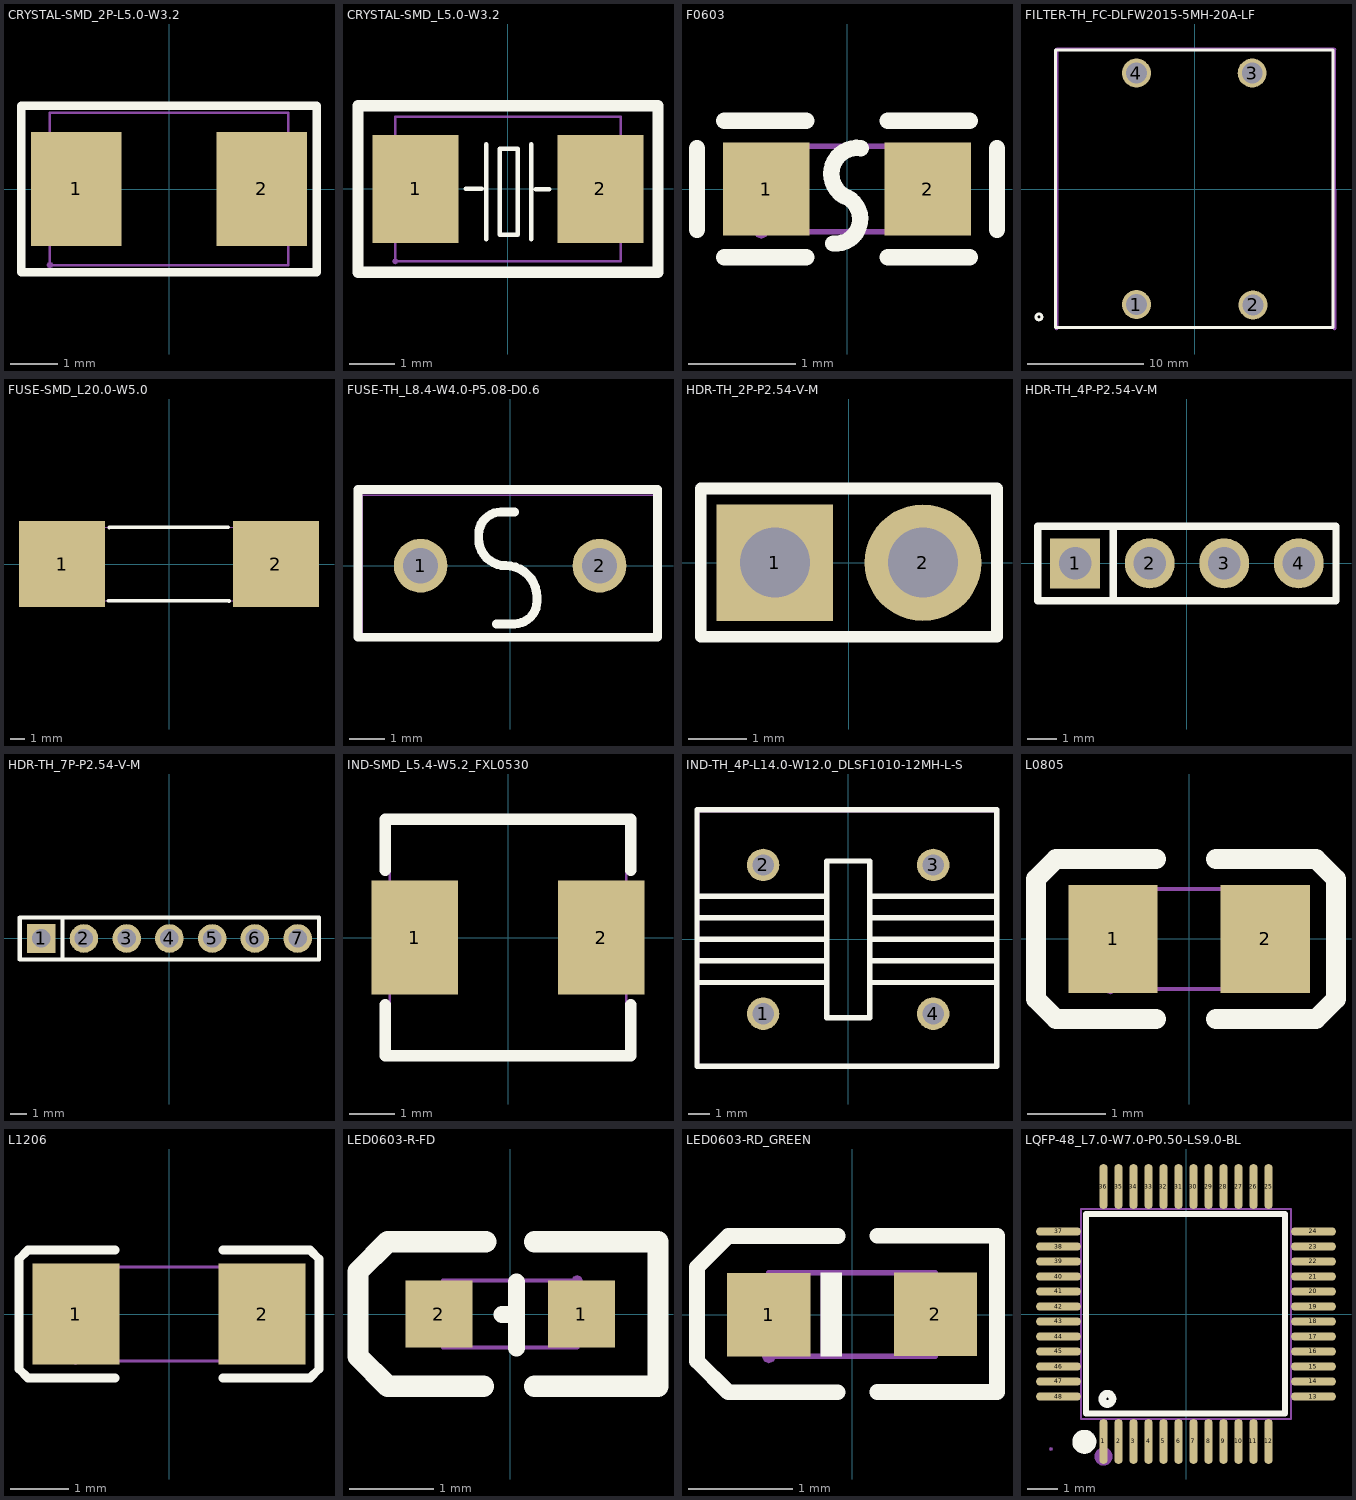
[diagram p0: the footprints below, top view; thin cyan lines are the x and y axes]
# Altium footprint library MISC84429-11.PcbLib: 64 footprints (part 2 of 4)
Each footprint in its own frame and in the unit in brackets; x right, y up, seen from the top. Pads: shape width x height; smd on the part's side, far side on the other; paste and mask are expansions set on the pad; w line width, h text height; cw(c..) or ccw(c..) is an arc to the next point about the centre after c.

## CRYSTAL-SMD_2P-L5.0-W3.2 [mm]
pads (2):
  rect 1.9x2.4 smd: 1(-1.95,0) 2(1.95,0)
Top Overlay:
  lines w0.18: -3.099,-1.75 3.099,-1.75 3.099,1.75 -3.099,1.75 -3.099,1.4 -3.099,-1.75
Mechanical 2:
  region: -2.435,-1.6 -2.454,-1.646 -2.5,-1.665 -2.546,-1.646 -2.565,-1.6 -2.546,-1.554 -2.5,-1.535 -2.454,-1.554
  region: 1.2,-1 1.2,1 2.5,1 2.5,-1
  region: -1.2,-1 -1.2,1 -2.5,1 -2.5,-1
  lines w0.051: -2.5,-1.6 -2.5,1.6 2.5,1.6 2.5,-1.6 -2.5,-1.6

## CRYSTAL-SMD_L5.0-W3.2 [mm]
pads (2):
  rect 1.9x2.4 smd: 1(-2.05,0) 2(2.05,0)
Top Overlay:
  lines w0.1: -0.94,0 -0.584,0 ; -0.483,-1.109 -0.483,0.991 ; 0.517,-1.109 0.517,0.991 ; 0.617,-0.009 0.917,-0.009 ; -0.183,-1.009 -0.183,0.89 0.217,0.89 0.217,-1.009 -0.183,-1.009
  lines w0.254: -3.325,-1.85 3.325,-1.85 3.325,-0.7 3.325,0.7 3.325,1.85 -3.325,1.85 -3.325,0.7 -3.325,-0.7 -3.325,-1.85
Mechanical 2:
  region: -2.435,-1.6 -2.454,-1.646 -2.5,-1.665 -2.546,-1.646 -2.565,-1.6 -2.546,-1.554 -2.5,-1.535 -2.454,-1.554
  region: -2.4,1 -1.3,1 -1.3,-1 -2.4,-1
  region: 1.3,1 2.4,1 2.4,-1 1.3,-1
  lines w0.051: -2.5,-1.6 -2.5,1.6 2.5,1.6 2.5,-1.6 -2.5,-1.6

## F0603 [mm]
pads (2):
  rect 0.806x0.864 smd paste-100 mask+0.051: 1(-0.753,0) 2(0.753,0)
Top Overlay:
  lines w0.152: -1.397,-0.381 -1.397,0.381 ; -1.143,-0.635 -0.381,-0.635 ; -1.143,0.635 -0.381,0.635 ; -0.127,-0.508 ccw(c-0.107,-0.28) -0.031,-0.063 ; -0.032,-0.064 cw(c0.096,0.142) 0.127,0.381 ; 0.381,-0.635 1.143,-0.635 ; 0.381,0.635 1.143,0.635 ; 1.397,-0.381 1.397,0.381
Top Paste:
  region: 0.315,-0.138 0.315,0.138 0.589,0.432 1.092,0.432 1.156,0.368 1.156,-0.368 1.092,-0.432 0.589,-0.432
  region: -0.315,-0.138 -0.315,0.138 -0.589,0.432 -1.092,0.432 -1.156,0.368 -1.156,-0.368 -1.092,-0.432 -0.589,-0.432
Mechanical 2:
  region: -0.735,-0.4 -0.754,-0.446 -0.8,-0.465 -0.846,-0.446 -0.865,-0.4 -0.846,-0.354 -0.8,-0.335 -0.754,-0.354
  region: -0.8,-0.4 -0.8,0.4 -0.5,0.4 -0.5,-0.4
  region: 0.8,-0.4 0.8,0.4 0.5,0.4 0.5,-0.4
  lines w0.051: -0.8,-0.4 -0.8,0.4 0.8,0.4 0.8,-0.4 -0.8,-0.4

## FILTER-TH_FC-DLFW2015-5MH-20A-LF [mm]
pads (4):
  round 2.5 hole 1.8 paste+0 mask-0.3: 1(-5.04,-9.983) 2(5.04,-10.016) 3(4.96,10.016) 4(-5.04,10.016)
Top Overlay:
  circle w0.254: c-13.462,-11.049 r0.254
  lines w0.254: -12.04,-11.983 11.96,-11.983 11.96,12.016 -12.04,12.016 -12.04,-11.983
Mechanical 1:
  region: -12.065,-12.065 -12.075,12.065 -12.035,12.162 -11.938,12.202 -11.938,12.192 12.065,12.202 12.162,12.162 12.202,12.065 12.192,12.065 12.202,-12.065 12.162,-12.162 12.065,-12.202 11.968,-12.162 11.928,-12.065 11.938,-12.065 11.938,11.938 -11.811,11.938 -11.801,-12.065 -11.841,-12.162 -11.938,-12.202 -12.035,-12.162 -12.075,-12.065
Mechanical 2:
  region: -4.284,-9.983 -4.309,-10.179 -4.385,-10.362 -4.505,-10.518 -4.662,-10.639 -4.844,-10.714 -5.04,-10.74 -5.236,-10.714 -5.418,-10.639 -5.575,-10.518 -5.695,-10.362 -5.771,-10.179 -5.796,-9.983 -5.771,-9.788 -5.695,-9.605 -5.575,-9.449 -5.418,-9.328 -5.236,-9.253 -5.04,-9.227 -4.844,-9.253 -4.662,-9.328 -4.505,-9.449 -4.385,-9.605 -4.309,-9.788
  region: 5.796,-10.016 5.771,-10.212 5.695,-10.395 5.575,-10.551 5.418,-10.672 5.236,-10.747 5.04,-10.773 4.844,-10.747 4.662,-10.672 4.505,-10.551 4.385,-10.395 4.309,-10.212 4.284,-10.016 4.309,-9.821 4.385,-9.638 4.505,-9.482 4.662,-9.361 4.844,-9.286 5.04,-9.26 5.236,-9.286 5.418,-9.361 5.575,-9.482 5.695,-9.638 5.771,-9.821
  region: 5.716,10.016 5.691,9.821 5.615,9.638 5.495,9.482 5.338,9.361 5.156,9.286 4.96,9.26 4.764,9.286 4.582,9.361 4.425,9.482 4.305,9.638 4.229,9.821 4.204,10.016 4.229,10.212 4.305,10.395 4.425,10.551 4.582,10.672 4.764,10.747 4.96,10.773 5.156,10.747 5.338,10.672 5.495,10.551 5.615,10.395 5.691,10.212
  region: -4.284,10.016 -4.309,9.821 -4.385,9.638 -4.505,9.482 -4.662,9.361 -4.844,9.286 -5.04,9.26 -5.236,9.286 -5.418,9.361 -5.575,9.482 -5.695,9.638 -5.771,9.821 -5.796,10.016 -5.771,10.212 -5.695,10.395 -5.575,10.551 -5.418,10.672 -5.236,10.747 -5.04,10.773 -4.844,10.747 -4.662,10.672 -4.505,10.551 -4.385,10.395 -4.309,10.212
  region: -11.935,-12 -11.954,-12.046 -12,-12.065 -12.046,-12.046 -12.065,-12 -12.046,-11.954 -12,-11.935 -11.954,-11.954
  lines w0.051: -12,-12 -12,12 12,12 12,-12 -12,-12

## FUSE-SMD_L20.0-W5.0 [mm]
pads (2):
  rect 6x6 smd: 1(-7.45,0) 2(7.45,0)
Top Overlay:
  lines w0.254: -4.219,-2.561 4.175,-2.58 ; -4.167,2.54 4.139,2.549
Mechanical 2:
  region: -9.935,-2.6 -9.954,-2.646 -10,-2.665 -10.046,-2.646 -10.065,-2.6 -10.046,-2.554 -10,-2.535 -9.954,-2.554
  region: 4.9,-2.6 4.9,2.6 10,2.6 10,-2.6
  region: -4.9,2.6 -4.9,-2.6 -10,-2.6 -10,2.6
  lines w0.051: -10,-2.56 10,-2.56 10,2.56 -10,2.56 -10,-2.56

## FUSE-TH_L8.4-W4.0-P5.08-D0.6 [mil]
pads (2):
  round 60 hole 39.37 paste+0 mask-8.35: 1(-100,0) 2(100,0)
Top Overlay:
  lines w10: -15,-65 5,-65 ccw(c5,-40) 30,-40 30,-35 ccw(c-5,-35) -5,0 cw(c-5,30) -35,30 -35,35 cw(c-10,35) -10,60 5,60 ; -170,-80 165,-80 165,85 -170,85 -170,-80
Mechanical 2:
  region: -162.79,-78.74 -163.54,-80.55 -165.35,-81.3 -167.16,-80.55 -167.91,-78.74 -167.16,-76.93 -165.35,-76.18 -163.54,-76.93
  region: 112.05,0 111.13,-4.61 108.52,-8.52 104.61,-11.13 100,-12.05 95.39,-11.13 91.48,-8.52 88.87,-4.61 87.95,0 88.87,4.61 91.48,8.52 95.39,11.13 100,12.05 104.61,11.13 108.52,8.52 111.13,4.61
  region: -87.95,0 -88.87,-4.61 -91.48,-8.52 -95.39,-11.13 -100,-12.05 -104.61,-11.13 -108.52,-8.52 -111.13,-4.61 -112.05,0 -111.13,4.61 -108.52,8.52 -104.61,11.13 -100,12.05 -95.39,11.13 -91.48,8.52 -88.87,4.61
  lines w2: -165.35,-78.74 -165.35,78.74 165.35,78.74 165.35,-78.74 -165.35,-78.74

## HDR-TH_2P-P2.54-V-M [mm]
pads (2):
  rect 2x2 hole 1.2: 1(-1.27,0)
  round 2 hole 1.2: 2(1.27,0)
Top Overlay:
  lines w0.203: -2.54,-1.27 2.54,-1.27 2.54,1.27 -0.635,1.27 -2.54,1.27 -2.54,-1.27
Mechanical 2:
  region: -2.475,-1.25 -2.494,-1.296 -2.54,-1.315 -2.586,-1.296 -2.605,-1.25 -2.586,-1.204 -2.54,-1.185 -2.494,-1.204
  region: 0.95,0.32 1.59,0.32 1.59,-0.32 0.95,-0.32
  region: -1.59,0.32 -0.95,0.32 -0.95,-0.32 -1.59,-0.32
  lines w0.051: -2.54,-1.25 -2.54,1.25 2.54,1.25 2.54,-1.25 -2.54,-1.25

## HDR-TH_4P-P2.54-V-M [mm]
pads (4):
  rect 1.7x1.7 hole 1.1: 1(-3.81,0)
  round 1.7 hole 1.1: 2(-1.27,0) 3(1.27,0) 4(3.81,0)
Top Overlay:
  lines w0.254: -2.516,-1.27 -2.516,1.27 ; -2.516,1.27 5.08,1.27 5.08,-1.27 -5.08,-1.27 -5.08,1.27 -2.516,1.27
Mechanical 2:
  region: -5.015,-1.25 -5.034,-1.296 -5.08,-1.315 -5.126,-1.296 -5.145,-1.25 -5.126,-1.204 -5.08,-1.185 -5.034,-1.204
  region: -4.13,0.32 -3.49,0.32 -3.49,-0.32 -4.13,-0.32
  region: -1.59,0.32 -0.95,0.32 -0.95,-0.32 -1.59,-0.32
  region: 0.95,0.32 1.59,0.32 1.59,-0.32 0.95,-0.32
  region: 3.49,0.32 4.13,0.32 4.13,-0.32 3.49,-0.32
  lines w0.051: -5.08,-1.25 -5.08,1.25 5.08,1.25 5.08,-1.25 -5.08,-1.25

## HDR-TH_7P-P2.54-V-M [mm]
pads (7):
  rect 1.7x1.7 hole 1.1: 1(-7.62,0)
  round 1.7 hole 1.1: 2(-5.08,0) 3(-2.54,0) 4(0,0) 5(2.54,0) 6(5.08,0) 7(7.62,0)
Top Overlay:
  lines w0.254: -6.35,-1.25 -6.35,1.25 ; -8.89,-1.25 8.89,-1.25 8.89,1.25 -8.89,1.25 -8.89,-1.25
Mechanical 2:
  region: -8.81,-1.25 -8.829,-1.296 -8.875,-1.315 -8.921,-1.296 -8.94,-1.25 -8.921,-1.204 -8.875,-1.185 -8.829,-1.204
  region: 7.3,0.32 7.94,0.32 7.94,-0.32 7.3,-0.32
  region: 4.76,0.32 5.4,0.32 5.4,-0.32 4.76,-0.32
  region: 2.22,0.32 2.86,0.32 2.86,-0.32 2.22,-0.32
  region: -0.32,0.32 0.32,0.32 0.32,-0.32 -0.32,-0.32
  region: -2.86,0.32 -2.22,0.32 -2.22,-0.32 -2.86,-0.32
  region: -5.4,0.32 -4.76,0.32 -4.76,-0.32 -5.4,-0.32
  region: -7.94,0.32 -7.3,0.32 -7.3,-0.32 -7.94,-0.32
  lines w0.051: -8.89,-1.25 -8.89,1.25 8.89,1.25 8.89,-1.25 -8.89,-1.25

## IND-SMD_L5.4-W5.2_FXL0530 [mm]
pads (2):
  rect 1.9x2.5 smd: 1(-2.05,0) 2(2.05,0)
Top Overlay:
  lines w0.254: -2.7,-1.481 -2.7,-2.6 2.7,-2.6 2.7,-1.481 ; -2.7,1.481 -2.7,2.6 2.7,2.6 2.7,1.481
Mechanical 2:
  region: -2.635,-2.6 -2.654,-2.646 -2.7,-2.665 -2.746,-2.646 -2.765,-2.6 -2.746,-2.554 -2.7,-2.535 -2.654,-2.554
  region: -2.7,1.1 -1.5,1.1 -1.5,-1.1 -2.7,-1.1
  region: 2.7,-1.1 1.5,-1.1 1.5,1.1 2.7,1.1
  lines w0.051: -2.6,-2.6 2.6,-2.6 2.6,2.6 -2.6,2.6 -2.6,-2.6

## IND-TH_4P-L14.0-W12.0_DLSF1010-12MH-L-S [mm]
pads (4):
  round 1.524 hole 1 paste+0 mask-0.212: 1(-4,-3.5) 2(-4,3.5) 3(4,3.5) 4(4,-3.5)
Top Overlay:
  lines w0.254: -7.112,0 -1.016,0 ; -6.985,-2.032 -1.016,-2.032 ; -6.985,-1.016 -1.016,-1.016 ; -6.985,1.016 -1.016,1.016 ; -6.985,2.032 -1.016,2.032 ; 1.016,-2.032 6.985,-2.032 ; 1.016,-1.016 6.985,-1.016 ; 1.016,0 6.731,0 6.985,0 ; 1.016,1.016 6.858,1.016 ; 1.016,2.032 6.985,2.032 ; -7.112,-5.969 6.985,-5.969 6.985,6.096 -7.112,6.096 -7.112,-5.969 ; -1.016,-3.683 1.016,-3.683 1.016,3.683 -1.016,3.683 -1.016,-3.683
Mechanical 2:
  region: -6.935,-6 -6.954,-6.046 -7,-6.065 -7.046,-6.046 -7.065,-6 -7.046,-5.954 -7,-5.935 -6.954,-5.954
  region: 4.306,-3.5 4.283,-3.617 4.216,-3.716 4.117,-3.783 4,-3.806 3.883,-3.783 3.784,-3.716 3.717,-3.617 3.694,-3.5 3.717,-3.383 3.784,-3.284 3.883,-3.217 4,-3.194 4.117,-3.217 4.216,-3.284 4.283,-3.383
  region: -3.694,-3.5 -3.717,-3.617 -3.784,-3.716 -3.883,-3.783 -4,-3.806 -4.117,-3.783 -4.216,-3.716 -4.283,-3.617 -4.306,-3.5 -4.283,-3.383 -4.216,-3.284 -4.117,-3.217 -4,-3.194 -3.883,-3.217 -3.784,-3.284 -3.717,-3.383
  region: 4.306,3.5 4.283,3.383 4.216,3.284 4.117,3.217 4,3.194 3.883,3.217 3.784,3.284 3.717,3.383 3.694,3.5 3.717,3.617 3.784,3.716 3.883,3.783 4,3.806 4.117,3.783 4.216,3.716 4.283,3.617
  region: -3.694,3.5 -3.717,3.383 -3.784,3.284 -3.883,3.217 -4,3.194 -4.117,3.217 -4.216,3.284 -4.283,3.383 -4.306,3.5 -4.283,3.617 -4.216,3.716 -4.117,3.783 -4,3.806 -3.883,3.783 -3.784,3.716 -3.717,3.617
  lines w0.051: -7,-6 -7,6 7,6 7,-6 -7,-6

## L0805 [mm]
pads (2):
  rect 1.133x1.377 smd paste-100 mask+0.051: 1(-0.966,0) 2(0.966,0)
Top Overlay:
  lines w0.254: -0.421,-1.016 -1.691,-1.016 -1.945,-0.762 -1.945,-0.635 -1.945,0.762 -1.691,1.016 -1.564,1.016 -0.421,1.016 ; 0.341,-1.016 1.484,-1.016 1.611,-1.016 1.865,-0.762 1.865,0.635 1.865,0.762 1.611,1.016 0.341,1.016
Top Paste:
  region: -0.36,-0.22 -0.36,0.22 -0.745,0.689 -1.433,0.689 -1.533,0.589 -1.533,-0.588 -1.433,-0.688 -0.745,-0.688
  region: 0.36,-0.22 0.36,0.22 0.745,0.689 1.433,0.689 1.533,0.589 1.533,-0.588 1.433,-0.688 0.745,-0.688
Mechanical 2:
  region: -0.935,-0.637 -0.954,-0.683 -1,-0.702 -1.046,-0.683 -1.065,-0.637 -1.046,-0.592 -1,-0.573 -0.954,-0.592
  region: 1,-0.637 1,0.638 0.6,0.638 0.6,-0.637
  region: -1,-0.637 -1,0.638 -0.6,0.638 -0.6,-0.637
  lines w0.051: -1,-0.637 -1,0.638 1,0.638 1,-0.637 -1,-0.637

## L1206 [mm]
pads (2):
  rect 1.485x1.728 smd paste-100 mask+0.051: 1(-1.593,0) 2(1.593,0)
Top Overlay:
  lines w0.152: -0.926,-1.093 -2.411,-1.093 -2.564,-0.94 -2.564,0.94 -2.411,1.093 -0.926,1.093 ; 0.926,-1.093 2.411,-1.093 2.564,-0.94 2.564,0.94 2.411,1.093 0.926,1.093
Top Paste:
  region: 0.85,-0.764 0.85,-0.394 0.95,-0.294 1.255,-0.294 1.355,-0.194 1.355,0.194 1.255,0.294 0.95,0.294 0.85,0.394 0.85,0.764 0.95,0.864 2.235,0.864 2.335,0.764 2.335,-0.764 2.235,-0.864 0.95,-0.864
  region: -0.85,-0.764 -0.85,-0.394 -0.95,-0.294 -1.255,-0.294 -1.355,-0.194 -1.355,0.194 -1.255,0.294 -0.95,0.294 -0.85,0.394 -0.85,0.764 -0.95,0.864 -2.235,0.864 -2.335,0.764 -2.335,-0.764 -2.235,-0.864 -0.95,-0.864
Mechanical 2:
  region: -1.535,-0.8 -1.554,-0.846 -1.6,-0.865 -1.646,-0.846 -1.665,-0.8 -1.646,-0.754 -1.6,-0.735 -1.554,-0.754
  region: -1.6,-0.8 -1.6,0.8 -1.1,0.8 -1.1,-0.8
  region: 1.6,-0.8 1.6,0.8 1.1,0.8 1.1,-0.8
  lines w0.051: -1.6,-0.8 -1.6,0.8 1.6,0.8 1.6,-0.8 -1.6,-0.8

## LED0603-R-FD [mm]
pads (2):
  rect 0.8x0.8 smd: 1(0.851,0) 2(-0.851,0)
Top Overlay:
  lines w0.203: -0.099,-0.008 0.076,-0.008 ; 0.076,-0.406 0.076,0.381
  lines w0.254: -0.318,-0.864 -1.46,-0.864 -1.816,-0.508 -1.816,0.508 -1.46,0.864 -0.292,0.864 ; 0.292,-0.864 1.765,-0.864 1.765,0.864 0.292,0.864
Mechanical 1:
  region: 1.225,-0.069 0.564,-0.069 0.564,0.083 1.225,0.083
  region: 0.988,0.35 0.988,-0.311 0.835,-0.311 0.835,0.35
  region: -0.508,-0.074 -1.168,-0.074 -1.168,0.078 -0.508,0.078
Mechanical 2:
  region: 0.865,0.4 0.846,0.354 0.8,0.335 0.754,0.354 0.735,0.4 0.754,0.446 0.8,0.465 0.846,0.446
  region: -0.8,-0.4 -0.8,0.4 -0.5,0.4 -0.5,-0.4
  region: 0.8,0.4 0.8,-0.4 0.5,-0.4 0.5,0.4
  lines w0.051: -0.8,-0.4 0.8,-0.4 0.8,0.4 -0.8,0.4 -0.8,-0.4

## LED0603-RD_GREEN [mm]
pads (2):
  rect 0.8x0.8 smd: 1(-0.799,-0.003) 2(0.799,0.003)
Top Overlay:
  region: -0.3,0.4 -0.3,-0.4 -0.1,-0.4 -0.1,0.4
  lines w0.15: -0.14,-0.746 -1.19,-0.746 -1.49,-0.446 -1.49,-0.346 -1.49,0.354 -1.49,0.454 -1.19,0.754 -0.14,0.754 ; 0.24,-0.744 1.39,-0.744 ; 0.24,0.757 1.39,0.757 1.39,-0.723
Mechanical 1:
  region: 0.529,0.068 1.069,0.068 1.069,-0.062 0.529,-0.062
  region: 0.735,-0.267 0.735,0.273 0.865,0.273 0.865,-0.267
  region: -1.07,0.062 -0.53,0.062 -0.53,-0.068 -1.07,-0.068
  region: -0.3,0.4 -0.3,-0.4 -0.1,-0.4 -0.1,0.4
Mechanical 2:
  region: -0.735,-0.403 -0.754,-0.449 -0.8,-0.468 -0.845,-0.449 -0.865,-0.403 -0.845,-0.358 -0.8,-0.339 -0.754,-0.358
  region: 0.5,-0.396 0.5,0.404 0.8,0.404 0.8,-0.396
  region: -0.8,-0.403 -0.8,0.397 -0.5,0.397 -0.5,-0.403
  lines w0.051: -0.8,-0.4 -0.8,0.4 0.8,0.4 0.8,-0.4 -0.8,-0.4

## LQFP-48_L7.0-W7.0-P0.50-LS9.0-BL [mm]
pads (48):
  oval 0.27x1.5 smd paste+0 mask+0.05: 1(-2.75,-4.25) 2(-2.25,-4.25) 3(-1.75,-4.25) 4(-1.25,-4.25) 5(-0.75,-4.25) 6(-0.25,-4.25) 7(0.25,-4.25) 8(0.75,-4.25) 9(1.25,-4.25) 10(1.75,-4.25) 11(2.25,-4.25) 12(2.75,-4.25) 25(2.75,4.25) 26(2.25,4.25) 27(1.75,4.25) 28(1.25,4.25) 29(0.75,4.25) 30(0.25,4.25) 31(-0.25,4.25) 32(-0.75,4.25) 33(-1.25,4.25) 34(-1.75,4.25) 35(-2.25,4.25) 36(-2.75,4.25)
  oval 1.5x0.27 smd paste+0 mask+0.05: 13(4.25,-2.75) 14(4.25,-2.25) 15(4.25,-1.75) 16(4.25,-1.25) 17(4.25,-0.75) 18(4.25,-0.25) 19(4.25,0.25) 20(4.25,0.75) 21(4.25,1.25) 22(4.25,1.75) 23(4.25,2.25) 24(4.25,2.75) 37(-4.25,2.75) 38(-4.25,2.25) 39(-4.25,1.75) 40(-4.25,1.25) 41(-4.25,0.75) 42(-4.25,0.25) 43(-4.25,-0.25) 44(-4.25,-0.75) 45(-4.25,-1.25) 46(-4.25,-1.75) 47(-4.25,-2.25) 48(-4.25,-2.75)
Top Overlay:
  circle w0.254: c-2.62,-2.83 r0.17
  lines w0.2: -2.896,3.34 3.302,3.34 3.302,-3.315 -3.327,-3.315 -3.327,3.34 -2.565,3.34
  lines w0.4: -3.39,-4.06 ccw(c-3.389,-4.26) -3.387,-4.06
Mechanical 1:
  circle w0.3: c-2.75,-4.75 r0.15
Mechanical 2:
  drawing of 101 lines, arcs and shapes, not listed